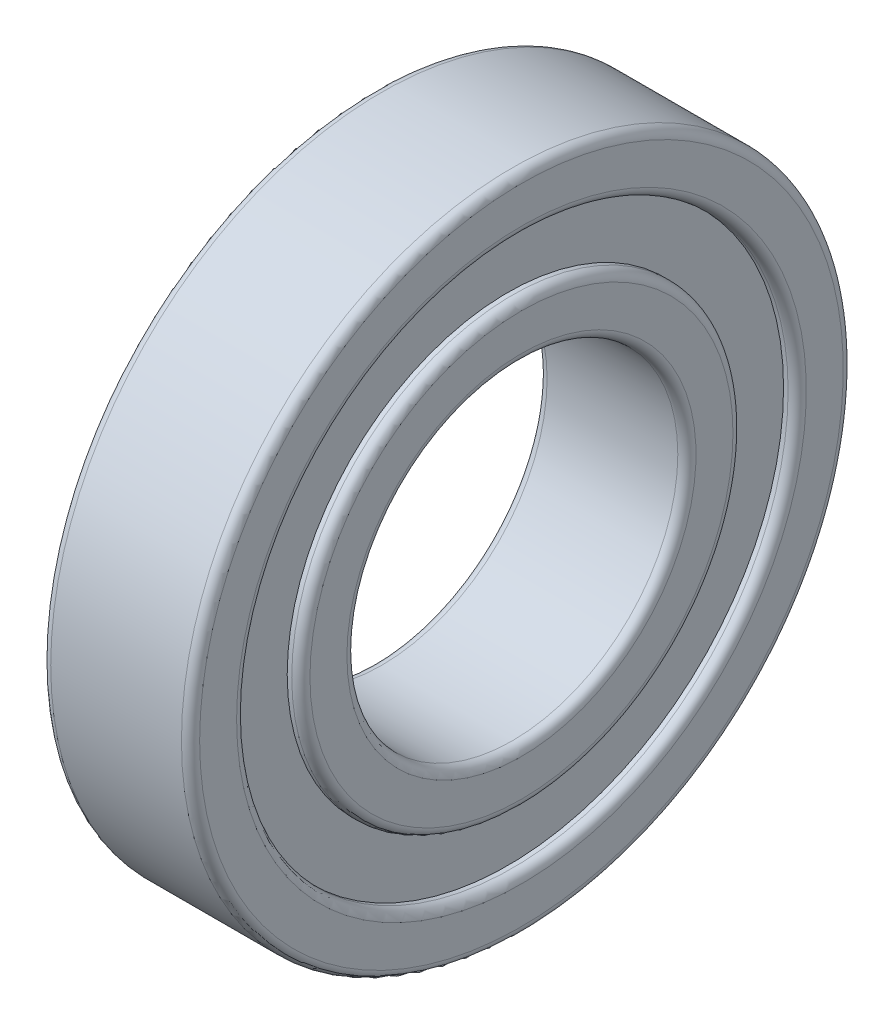
from build123d import *

# Parameters (mm, degrees)
SKETCH_5_W               = 3
SKETCH_5_H               = 2.000000000000007
PATTERN_CIRCULAR_5_COUNT = 15
PATTERN_CIRCULAR_2_COUNT = 15
SKETCH_8_W               = 1.1000000000000014
SKETCH_8_H               = 8.866666666666664


with BuildPart() as part:
    # 草图2 → 旋转1 (revolve)
    with BuildSketch(Plane.XY, mode=Mode.PRIVATE) as revolve_1_sk:
        with BuildLine():
            Line((7.9, 19.999999999999996), (-7.9, 19.999999999999996))
            ThreePointArc((-7.9, 19.999999999999996), (-8.677817459305205, 20.322182540694797), (-9.000000000000002, 21.1))
            Line((-9.000000000000002, 21.1), (-9, 25.56666666666666))
            ThreePointArc((-9, 25.56666666666666), (-8.6778174593052, 26.34448412597186), (-7.9, 26.666666666666657))
            Line((-7.9, 26.666666666666657), (-3.726779962499638, 26.666666666666668))
            ThreePointArc((-3.726779962499638, 26.666666666666668), (7.3e-16, 25.000000000000007), (3.726779962499638, 26.666666666666668))
            Line((3.726779962499638, 26.666666666666668), (7.899999999999998, 26.666666666666664))
            ThreePointArc((7.899999999999998, 26.666666666666664), (8.677817459305201, 26.344484125971867), (9, 25.566666666666663))
            Line((9, 25.566666666666663), (9.000000000000002, 21.1))
            ThreePointArc((9.000000000000002, 21.1), (8.677817459305206, 20.322182540694797), (7.9, 19.999999999999996))
        make_face()
        with BuildLine():
            Line((-8.999999999999996, 38.900000000000006), (-9.000000000000005, 34.43333333333333))
            ThreePointArc((-9.000000000000005, 34.43333333333333), (-8.677817459305206, 33.655515874028126), (-7.8999999999999995, 33.33333333333333))
            Line((-7.8999999999999995, 33.33333333333333), (-3.7267799624996396, 33.33333333333333))
            ThreePointArc((-3.7267799624996396, 33.33333333333333), (7.3e-16, 34.999999999999986), (3.7267799624996396, 33.33333333333333))
            Line((3.7267799624996396, 33.33333333333333), (7.899999999999998, 33.33333333333333))
            ThreePointArc((7.899999999999998, 33.33333333333333), (8.677817459305201, 33.655515874028126), (9.000000000000002, 34.43333333333333))
            Line((9.000000000000002, 34.43333333333333), (8.999999999999993, 38.900000000000006))
            ThreePointArc((8.999999999999993, 38.900000000000006), (8.677817459305196, 39.6778174593052), (7.899999999999998, 40))
            Line((7.899999999999998, 40), (-7.9, 40))
            ThreePointArc((-7.9, 40), (-8.6778174593052, 39.6778174593052), (-8.999999999999996, 38.900000000000006))
        make_face()
    revolve(revolve_1_sk.sketch.rotate(Axis((-3.4999999999999996, 0, 0), (1, 0, 0)), 90), axis=Axis((-3.4999999999999996, 0, 0), (1, 0, 0)))


with BuildPart() as body_2:
    # 草图5 → 旋转3 (revolve)
    with BuildSketch(Plane.XY, mode=Mode.PRIVATE) as revolve_3_sk:
        with Locations((7.22e-15, 30)):
            Rectangle(SKETCH_5_W, SKETCH_5_H)
    revolve(revolve_3_sk.sketch.rotate(Axis((-19.927092192426834, 0, 0), (1, 0, 0)), 90), axis=Axis((-19.927092192426834, 0, 0), (1, 0, 0)))



with BuildPart() as body_3:
    # 草图3 → 旋转2 (revolve)
    with BuildSketch(Plane.XY):
        with BuildLine():
            Line((-5.4999999999999964, 30), (5.4999999999999964, 30))
            ThreePointArc((5.4999999999999964, 30), (2.98e-15, 35.49999999999999), (-5.4999999999999964, 30))
        make_face()
    revolve(axis=Axis((-5.4999999999999964, 30, 0), (1, 0, 0)))


with BuildPart() as pattern_circular_5_1:
    # 阵列(圆周)5: pattern copy
    add(body_3.part.rotate(Axis((0, -4e-16, 1.4e-16), (1, 0, 0)), 1 * 360 / PATTERN_CIRCULAR_5_COUNT))


with BuildPart() as pattern_circular_5_2:
    # 阵列(圆周)5: pattern copy
    add(body_3.part.rotate(Axis((0, -4e-16, 1.4e-16), (1, 0, 0)), 2 * 360 / PATTERN_CIRCULAR_5_COUNT))


with BuildPart() as pattern_circular_5_3:
    # 阵列(圆周)5: pattern copy
    add(body_3.part.rotate(Axis((0, -4e-16, 1.4e-16), (1, 0, 0)), 3 * 360 / PATTERN_CIRCULAR_5_COUNT))


with BuildPart() as pattern_circular_5_4:
    # 阵列(圆周)5: pattern copy
    add(body_3.part.rotate(Axis((0, -4e-16, 1.4e-16), (1, 0, 0)), 4 * 360 / PATTERN_CIRCULAR_5_COUNT))


with BuildPart() as pattern_circular_5_5:
    # 阵列(圆周)5: pattern copy
    add(body_3.part.rotate(Axis((0, -4e-16, 1.4e-16), (1, 0, 0)), 5 * 360 / PATTERN_CIRCULAR_5_COUNT))


with BuildPart() as pattern_circular_5_6:
    # 阵列(圆周)5: pattern copy
    add(body_3.part.rotate(Axis((0, -4e-16, 1.4e-16), (1, 0, 0)), 6 * 360 / PATTERN_CIRCULAR_5_COUNT))


with BuildPart() as pattern_circular_5_7:
    # 阵列(圆周)5: pattern copy
    add(body_3.part.rotate(Axis((0, -4e-16, 1.4e-16), (1, 0, 0)), 7 * 360 / PATTERN_CIRCULAR_5_COUNT))


with BuildPart() as pattern_circular_5_8:
    # 阵列(圆周)5: pattern copy
    add(body_3.part.rotate(Axis((0, -4e-16, 1.4e-16), (1, 0, 0)), 8 * 360 / PATTERN_CIRCULAR_5_COUNT))


with BuildPart() as pattern_circular_5_9:
    # 阵列(圆周)5: pattern copy
    add(body_3.part.rotate(Axis((0, -4e-16, 1.4e-16), (1, 0, 0)), 9 * 360 / PATTERN_CIRCULAR_5_COUNT))


with BuildPart() as pattern_circular_5_10:
    # 阵列(圆周)5: pattern copy
    add(body_3.part.rotate(Axis((0, -4e-16, 1.4e-16), (1, 0, 0)), 10 * 360 / PATTERN_CIRCULAR_5_COUNT))


with BuildPart() as pattern_circular_5_11:
    # 阵列(圆周)5: pattern copy
    add(body_3.part.rotate(Axis((0, -4e-16, 1.4e-16), (1, 0, 0)), 11 * 360 / PATTERN_CIRCULAR_5_COUNT))


with BuildPart() as pattern_circular_5_12:
    # 阵列(圆周)5: pattern copy
    add(body_3.part.rotate(Axis((0, -4e-16, 1.4e-16), (1, 0, 0)), 12 * 360 / PATTERN_CIRCULAR_5_COUNT))


with BuildPart() as pattern_circular_5_13:
    # 阵列(圆周)5: pattern copy
    add(body_3.part.rotate(Axis((0, -4e-16, 1.4e-16), (1, 0, 0)), 13 * 360 / PATTERN_CIRCULAR_5_COUNT))


with BuildPart() as pattern_circular_5_14:
    # 阵列(圆周)5: pattern copy
    add(body_3.part.rotate(Axis((0, -4e-16, 1.4e-16), (1, 0, 0)), 14 * 360 / PATTERN_CIRCULAR_5_COUNT))


with BuildPart() as cut_revolve_1_tool:
    # 草图6 → 切除-旋转1 (revolve)
    with BuildSketch(Plane.XY):
        with BuildLine():
            Line((-5.408326913195981, 31), (5.408326913195981, 31))
            ThreePointArc((5.408326913195981, 31), (1.76e-15, 35.49999999999999), (-5.408326913195981, 31))
        make_face()
        with BuildLine():
            Line((-5.408326913195981, 28.999999999999996), (5.408326913195981, 28.999999999999996))
            ThreePointArc((5.408326913195981, 28.999999999999996), (1.76e-15, 24.5), (-5.408326913195981, 28.999999999999996))
        make_face()
    revolve(axis=Axis((-19.927092192426834, 0, 0), (1, 0, 0)))


with BuildPart() as part_1:
    add(part.part)

    # 切除-旋转1: cut by cut_revolve_1_tool
    add(cut_revolve_1_tool.part, mode=Mode.SUBTRACT)

    # 草图8 → 旋转5 (revolve)
    with BuildSketch(Plane.XY, mode=Mode.PRIVATE) as revolve_5_sk:
        with Locations((6.799999999999999, 30)):
            Rectangle(SKETCH_8_W, SKETCH_8_H)
        Polygon((-6.249999999999986, 25.566666666666666), (-7.349999999999986, 25.566666666666663), (-7.34999999999999, 34.43333333333333), (-6.249999999999989, 34.43333333333333), align=None)
    revolve(revolve_5_sk.sketch.rotate(Axis((-19.927092192426834, 0, 0), (1, 0, 0)), 90), axis=Axis((-19.927092192426834, 0, 0), (1, 0, 0)))


with BuildPart() as body_3_1:
    add(body_3.part)

    # 切除-旋转1: cut by cut_revolve_1_tool
    add(cut_revolve_1_tool.part, mode=Mode.SUBTRACT)


with BuildPart() as pattern_circular_5_1_1:
    add(pattern_circular_5_1.part)

    # 切除-旋转1: cut by cut_revolve_1_tool
    add(cut_revolve_1_tool.part, mode=Mode.SUBTRACT)


with BuildPart() as pattern_circular_5_2_1:
    add(pattern_circular_5_2.part)

    # 切除-旋转1: cut by cut_revolve_1_tool
    add(cut_revolve_1_tool.part, mode=Mode.SUBTRACT)


with BuildPart() as pattern_circular_5_3_1:
    add(pattern_circular_5_3.part)

    # 切除-旋转1: cut by cut_revolve_1_tool
    add(cut_revolve_1_tool.part, mode=Mode.SUBTRACT)


with BuildPart() as pattern_circular_5_4_1:
    add(pattern_circular_5_4.part)

    # 切除-旋转1: cut by cut_revolve_1_tool
    add(cut_revolve_1_tool.part, mode=Mode.SUBTRACT)


with BuildPart() as pattern_circular_5_5_1:
    add(pattern_circular_5_5.part)

    # 切除-旋转1: cut by cut_revolve_1_tool
    add(cut_revolve_1_tool.part, mode=Mode.SUBTRACT)


with BuildPart() as pattern_circular_5_6_1:
    add(pattern_circular_5_6.part)

    # 切除-旋转1: cut by cut_revolve_1_tool
    add(cut_revolve_1_tool.part, mode=Mode.SUBTRACT)


with BuildPart() as pattern_circular_5_7_1:
    add(pattern_circular_5_7.part)

    # 切除-旋转1: cut by cut_revolve_1_tool
    add(cut_revolve_1_tool.part, mode=Mode.SUBTRACT)


with BuildPart() as pattern_circular_5_8_1:
    add(pattern_circular_5_8.part)

    # 切除-旋转1: cut by cut_revolve_1_tool
    add(cut_revolve_1_tool.part, mode=Mode.SUBTRACT)


with BuildPart() as pattern_circular_5_9_1:
    add(pattern_circular_5_9.part)

    # 切除-旋转1: cut by cut_revolve_1_tool
    add(cut_revolve_1_tool.part, mode=Mode.SUBTRACT)


with BuildPart() as pattern_circular_5_10_1:
    add(pattern_circular_5_10.part)

    # 切除-旋转1: cut by cut_revolve_1_tool
    add(cut_revolve_1_tool.part, mode=Mode.SUBTRACT)


with BuildPart() as pattern_circular_5_11_1:
    add(pattern_circular_5_11.part)

    # 切除-旋转1: cut by cut_revolve_1_tool
    add(cut_revolve_1_tool.part, mode=Mode.SUBTRACT)


with BuildPart() as pattern_circular_5_12_1:
    add(pattern_circular_5_12.part)

    # 切除-旋转1: cut by cut_revolve_1_tool
    add(cut_revolve_1_tool.part, mode=Mode.SUBTRACT)


with BuildPart() as pattern_circular_5_13_1:
    add(pattern_circular_5_13.part)

    # 切除-旋转1: cut by cut_revolve_1_tool
    add(cut_revolve_1_tool.part, mode=Mode.SUBTRACT)


with BuildPart() as pattern_circular_5_14_1:
    add(pattern_circular_5_14.part)

    # 切除-旋转1: cut by cut_revolve_1_tool
    add(cut_revolve_1_tool.part, mode=Mode.SUBTRACT)


with BuildPart() as body_2_1:
    add(body_2.part)

    add(body_3_1.part)  # 旋转4 merges body 3
    # 草图7 → 旋转4 (revolve)
    with BuildSketch(Plane.XY):
        with BuildLine():
            Line((-4.999999999999988, 30), (4.999999999999988, 30))
            ThreePointArc((4.999999999999988, 30), (2.95e-15, 34.999999999999986), (-4.999999999999988, 30))
        make_face()
    revolve_4 = revolve(axis=Axis((-4.999999999999988, 30, 0), (1, 0, 0)))

    # 阵列(圆周)2: 旋转4 ×15 about axis
    pattern_circular_2_axis = Axis((0, -4e-16, 1.4e-16), (1, 0, 0))
    for i in range(1, PATTERN_CIRCULAR_2_COUNT):
        add(revolve_4.rotate(pattern_circular_2_axis, i * 360 / PATTERN_CIRCULAR_2_COUNT))


solid = Compound([part_1.part, pattern_circular_5_1_1.part, pattern_circular_5_2_1.part, pattern_circular_5_3_1.part, pattern_circular_5_4_1.part, pattern_circular_5_5_1.part, pattern_circular_5_6_1.part, pattern_circular_5_7_1.part, pattern_circular_5_8_1.part, pattern_circular_5_9_1.part, pattern_circular_5_10_1.part, pattern_circular_5_11_1.part, pattern_circular_5_12_1.part, pattern_circular_5_13_1.part, pattern_circular_5_14_1.part, body_2_1.part])
